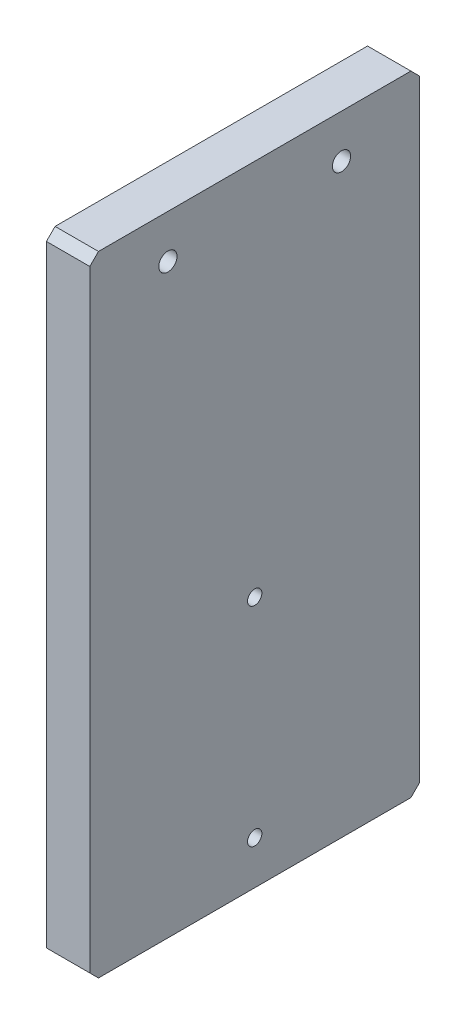
from build123d import *

# Parameters (mm, degrees)
SKETCH_1_W         = 76
SKETCH_1_H         = 145
EXTRUDE_1_DEPTH    = 10
HOLE_WIZARD_M5_1_D = 4.2
HOLE_WIZARD_M4_1_D = 3.3
CHAMFER_1_SIZE     = 2


with BuildPart() as part:
    # 草图1 → 凸台-拉伸1 (new body)
    with BuildSketch(Plane(origin=(0, 0, 0), x_dir=(0, 0, -1), z_dir=(1, 0, 0))):
        Rectangle(SKETCH_1_W, SKETCH_1_H)
    extrude(amount=EXTRUDE_1_DEPTH)

    # M5 螺纹孔1 (through all)
    with Locations(Plane.ZY):
        with Locations((20, 62.5), (-20, 62.5)):
            Hole(HOLE_WIZARD_M5_1_D / 2)

    # M4 螺纹孔1 (through all)
    with Locations(Plane.ZY):
        with Locations((0, -14.5), (0, -62.5)):
            Hole(HOLE_WIZARD_M4_1_D / 2)

    # 倒角1
    chamfer_1_edges = [part.edges().sort_by_distance(p)[0] for p in [
        (5, -72.5, -38),
        (5, -72.5, 38),
        (5, 72.5, 38),
        (5, 72.5, -38),
    ]]
    chamfer(chamfer_1_edges, length=CHAMFER_1_SIZE)


solid = part.part
